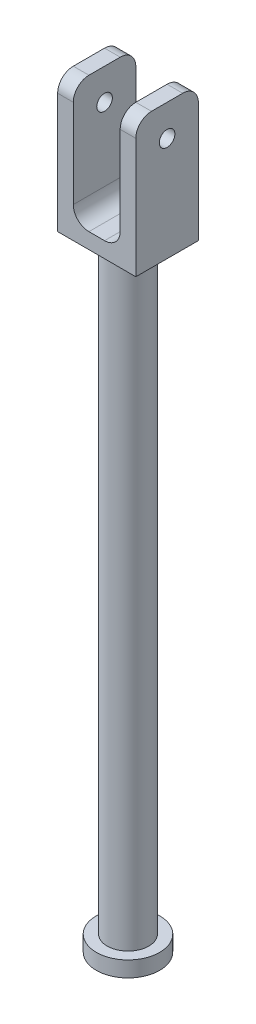
from build123d import *

# Parameters (mm, degrees)
BOSS_EXTRUDE1_DEPTH = 12
FILLET1_R           = 3
FILLET2_R           = 3
SKETCH2_R           = 1.5
CUT_EXTRUDE1_DEPTH  = 33.32645975
SKETCH3_R           = 4
BOSS_EXTRUDE2_DEPTH = 116
SKETCH4_R           = 6.081663029
BOSS_EXTRUDE3_DEPTH = 3


with BuildPart() as part:
    # Sketch1 → Boss-Extrude1 (new body)
    with BuildSketch(Plane.XY):
        Polygon((0, 26), (0, 0), (15, 0), (15, 26), (12, 26), (12, 3), (3, 3), (3, 26), align=None)
    extrude(amount=BOSS_EXTRUDE1_DEPTH)

    # Fillet1
    fillet1_edges = [part.edges().sort_by_distance(p)[0] for p in [
        (1.5, 26, 0),
        (13.5, 26, 12),
        (1.5, 26, 12),
        (13.5, 26, 0),
    ]]
    fillet(fillet1_edges, radius=FILLET1_R)

    # Fillet2
    fillet2_edges = [part.edges().sort_by_distance(p)[0] for p in [
        (3, 3, 6),
        (12, 3, 6),
    ]]
    fillet(fillet2_edges, radius=FILLET2_R)

    # Sketch2 → Cut-Extrude1 (cut, through all)
    with BuildSketch(Plane(origin=(15, 0, 0), x_dir=(0, 0, -1), z_dir=(1, 0, 0))):
        with Locations(Location((-6, 20, 0), (0, 0, 90))):
            Circle(SKETCH2_R)
    extrude(amount=-CUT_EXTRUDE1_DEPTH, mode=Mode.SUBTRACT)

    # Sketch3 → Boss-Extrude2 (add)
    with BuildSketch(Plane(origin=(0, 0, 0), x_dir=(-1, 0, 0), z_dir=(0, -1, 0))):
        with Locations(Location((-7.5, -6, 0), (0, 0, 270))):
            Circle(SKETCH3_R)
    extrude(amount=BOSS_EXTRUDE2_DEPTH)

    # Sketch4 → Boss-Extrude3 (add)
    with BuildSketch(Plane(origin=(0, -116, 0), x_dir=(-1, 0, 0), z_dir=(0, -1, 0))):
        with Locations(Location((-7.5, -6, 0), (0, 0, 90))):
            Circle(SKETCH4_R)
    extrude(amount=BOSS_EXTRUDE3_DEPTH)


solid = part.part
